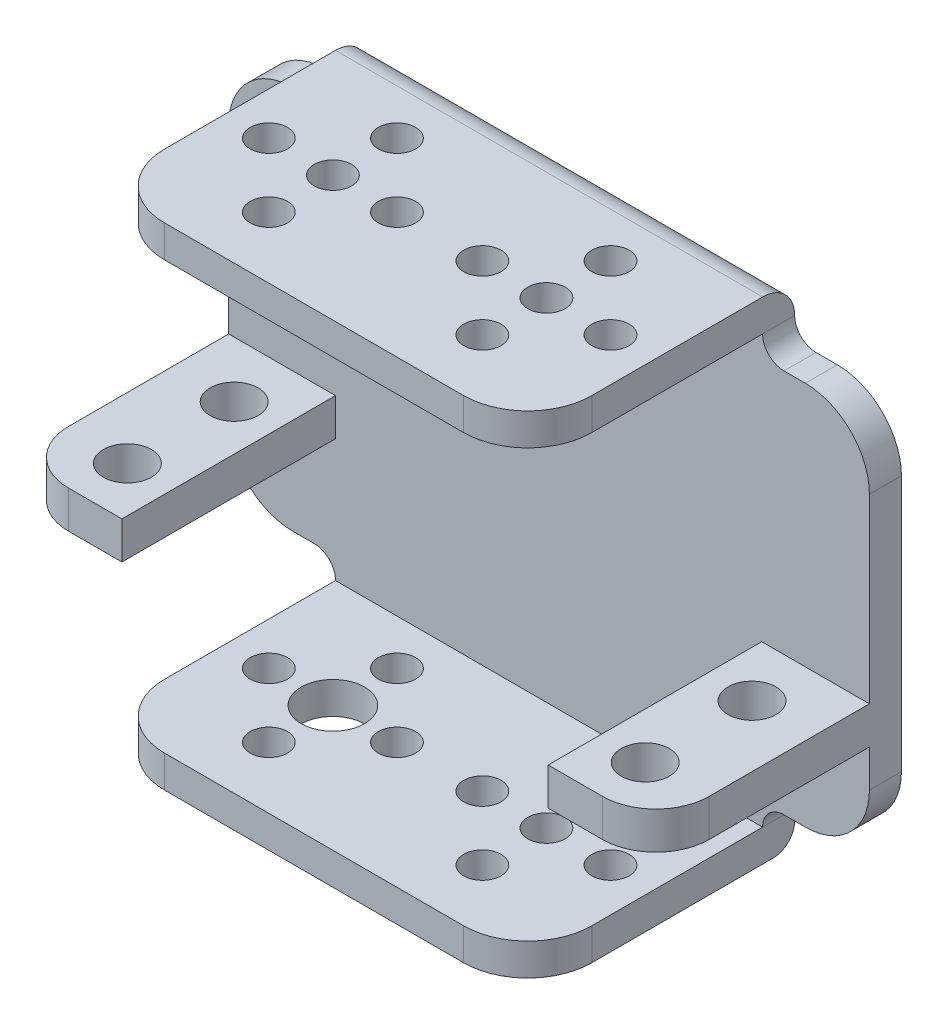
SolidWorks part; units mm, degrees
material "45"
ref_plane "Front Plane" through (0, 0, 0) normal (0, 0, 1) x (1, 0, 0)
ref_plane "Top Plane" through (0, 0, 0) normal (0, 1, 0) x (1, 0, 0)
ref_plane "Right Plane" through (0, 0, 0) normal (1, 0, 0) x (0, 0, -1)
sketch "Sketch1" plane through (0, 0, 0) normal (0, 0, 1) x (1, 0, 0)
  line L1 (-24.5297, 19.8459) -> (35.4703, 19.8459)
  line L2 (-24.5297, 19.8459) -> (-24.5297, -16.1541)
  line L3 (-24.5297, -16.1541) -> (35.4703, -16.1541)
  line L4 (35.4703, 19.8459) -> (35.4703, -16.1541)
  dimension "D1" = 60
  dimension "D2" = 36
extrude "Boss-Extrude1" add sketch "Sketch1" along normal blind 3
ref_plane "Plane1" through (0, 1.8459, 0) normal (0, -1, 0) x (-1, 0, 0)
ref_plane "Plane2" through (5.4703, 0, 0) normal (1, 0, 0) x (0, 0, -1)
sketch "Sketch3" plane through (5.4703, 0, 0) normal (1, 0, 0) x (0, 0, -1)
  line L0 (0, 22.8697) -> (0, 24.8459)
  line L1 (0, 24.8459) -> (-25, 24.8459)
  line L2 (-3, 19.8459) -> (0, 19.8459) construction
  line L3 (-25, 24.8459) -> (-25, 21.8459)
  line L4 (-25, 21.8459) -> (-3, 21.8459)
  line L5 (0, 22.8697) -> (0, 19.8459)
  line L6 (-3, 19.8459) -> (-3, 21.8459)
  line L7 (-3, 19.8459) -> (0, 19.8459)
  dimension "D1" = 25
  dimension "D2" = 5
  dimension "D3" = 3
extrude "Boss-Extrude2" add sketch "Sketch3" along normal mid plane 40
fillet "Fillet2" radius 3 1 edges at (5.4703, 24.8459, 0)
fillet "Fillet3" radius 2 2 edges
mirror "Mirror2" about plane through (0, 1.8459, 0) normal (0, -1, 0) of "Boss-Extrude2"
fillet "Fillet4" radius 2 2 edges
fillet "Fillet5" radius 2 1 edges at (5.4703, -21.1541, 0)
fillet "Fillet6" radius 6 4 edges at (-24.5297, -16.1541, 1.5) (-24.5297, 19.8459, 1.5) (35.4703, -16.1541, 1.5) (35.4703, 19.8459, 1.5)
fillet "Fillet7" radius 6 4 edges at (-14.5297, -19.6541, 25) (25.4703, -19.6541, 25) (25.4703, 23.3459, 25) (-14.5297, 23.3459, 25)
sketch "Sketch4" plane through (0, 24.8459, 0) normal (0, 1, 0) x (1, 0, 0)
  line L0 (25.4239, -7.8934) -> (25.4239, -18.5934) construction
  line L1 (19.4703, -25) -> (-8.5297, -25) construction
  circle A0 centre (15.4239, -13.2) radius 6 construction
  circle A1 centre (15.4239, -19.2) radius 1.75
  circle A2 centre (9.4239, -13.2) radius 1.75
  circle A3 centre (15.4239, -7.2) radius 1.75
  circle A4 centre (21.4239, -13.2) radius 1.75
  circle A5 centre (15.4239, -13.2) radius 1.75
  point P17 (15.4239, -13.2)
  dimension "D1" = 12
  dimension "D4" = 3.5
  dimension "D6" = 3.5
  dimension "D2" = 10
  dimension "D3" = 11.8
  dimension "D5" = 4
extrude "Cut-Extrude1" cut sketch "Sketch4" against normal through all
sketch "Sketch6" plane through (0, 0, 3) normal (0, 0, 1) x (1, 0, 0)
  line L0 (35.4703, -10.1541) -> (35.4703, 13.8459) construction
  line L1 (25.3868, -6.6541) -> (35.4703, -6.6541)
  line L2 (25.3868, -6.6541) -> (25.3868, -3.1541)
  line L3 (25.3868, -3.1541) -> (35.4703, -3.1541)
  line L4 (35.4703, -6.6541) -> (35.4703, -3.1541)
  line L5 (-24.5297, 13.8459) -> (-24.5297, -10.1541) construction
  line L6 (-14.5297, -6.6541) -> (-24.5297, -6.6541)
  line L7 (-14.5297, -6.6541) -> (-14.5297, -3.1541)
  line L8 (-14.5297, -3.1541) -> (-24.5297, -3.1541)
  line L9 (-24.5297, -6.6541) -> (-24.5297, -3.1541)
  dimension "D1" = 3.5
  dimension "D2" = 3.5
extrude "Boss-Extrude3" add sketch "Sketch6" along normal blind 20
fillet "Fillet8" radius 5 2 edges at (-24.5297, -4.9041, 23) (35.4703, -4.9041, 23)
sketch "Sketch7" plane through (0, -6.6541, 0) normal (0, -1, 0) x (1, 0, 0)
  circle A0 centre (29.7203, 18.2434) radius 2.25
  circle A1 centre (29.7203, 8.2434) radius 2.25
  circle A2 centre (-18.7797, 18.2434) radius 2.25
  circle A3 centre (-18.7797, 8.2434) radius 2.25
extrude "Cut-Extrude2" cut sketch "Sketch7" against normal through all
sketch "Sketch8" plane through (0, -21.1541, 0) normal (0, -1, 0) x (1, 0, 0)
  circle A0 centre (-4.5297, 13.2434) radius 2.97
extrude "Cut-Extrude3" cut sketch "Sketch8" against normal blind 20
sketch "Sketch9" plane through (0, -21.1541, 0) normal (0, -1, 0) x (1, 0, 0)
  circle A0 centre (-4.5297, 13.2434) radius 6 construction
  circle A1 centre (-4.5297, 19.2434) radius 1.75
  circle A2 centre (1.4703, 13.2434) radius 1.75
  circle A3 centre (-4.5297, 7.2434) radius 1.75
  circle A4 centre (-10.5297, 13.2434) radius 1.75
  point P14 (-4.5297, 13.2434)
  dimension "D1" = 12
  dimension "D2" = 3.5
  dimension "D3" = 4
extrude "Cut-Extrude4" cut sketch "Sketch9" against normal through all
sketch "Sketch10" plane through (0, 24.8459, 0) normal (0, 1, 0) x (1, 0, 0)
  circle A2 centre (-4.5297, -13.2434) radius 1.75
  dimension "D1" = 3.5
extrude "Cut-Extrude5" cut sketch "Sketch10" against normal blind 20
